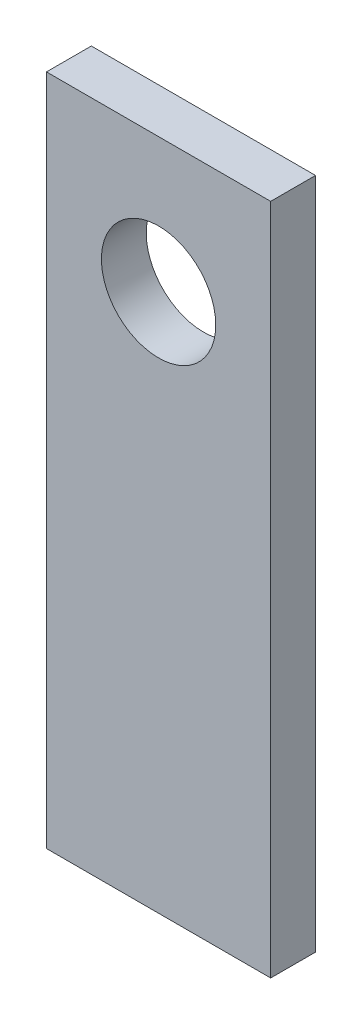
SolidWorks part; units mm, degrees
ref_plane "前视基准面" through (0, 0, 0) normal (0, 0, 1) x (1, 0, 0)
ref_plane "上视基准面" through (0, 0, 0) normal (0, 1, 0) x (1, 0, 0)
ref_plane "右视基准面" through (0, 0, 0) normal (1, 0, 0) x (0, 0, -1)
sketch "草图1" plane through (0, 0, 0) normal (0, 0, 1) x (1, 0, 0)
  line L1 (-25, -75) -> (25, -75)
  line L2 (-25, -75) -> (-25, 75)
  line L3 (-25, 75) -> (25, 75)
  line L4 (25, -75) -> (25, 75)
  line L5 (-25, -75) -> (25, 75) construction
  line L6 (-25, 75) -> (25, -75) construction
  point P0 (0, 0)
  dimension "D1" = 50
  dimension "D2" = 150
extrude "凸台-拉伸1" add sketch "草图1" along normal mid plane 10
sketch "草图2" plane through (0, 0, 5) normal (0, 0, 1) x (1, 0, 0)
  line L0 (25, 75) -> (-25, 75) construction
  circle A0 centre (0, 45) radius 12.75
  point P2 (0, 0)
  dimension "D1" = 25.5
  dimension "D2" = 30
extrude "切除-拉伸1" cut sketch "草图2" against normal up to next
